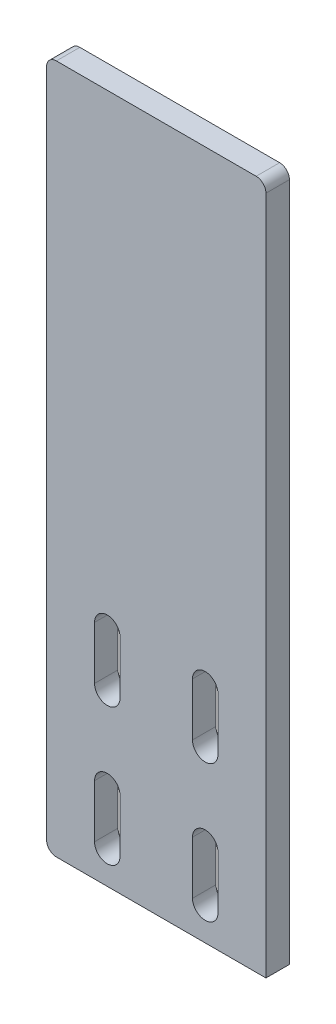
from build123d import *

# Parameters (mm, degrees)
SKETCH1_W           = 112
SKETCH1_H           = 352
BOSS_EXTRUDE1_DEPTH = 12
FILLET1_R           = 5


with BuildPart() as part:
    # Sketch1 → Boss-Extrude1 (new body)
    with BuildSketch(Plane.XY):
        Rectangle(SKETCH1_W, SKETCH1_H)
        with BuildLine():
            Line((-18.5, -62.5), (-18.5, -89.5))
            ThreePointArc((-18.5, -89.5), (-25, -96), (-31.5, -89.5))
            Line((-31.5, -89.5), (-31.5, -62.5))
            ThreePointArc((-31.5, -62.5), (-25, -56), (-18.5, -62.5))
        make_face(mode=Mode.SUBTRACT)
        with BuildLine():
            Line((31.5, -62.5), (31.5, -89.5))
            ThreePointArc((31.5, -89.5), (25, -96), (18.5, -89.5))
            Line((18.5, -89.5), (18.5, -62.5))
            ThreePointArc((18.5, -62.5), (25, -56), (31.5, -62.5))
        make_face(mode=Mode.SUBTRACT)
        with BuildLine():
            Line((-31.5, -132.5), (-31.5, -159.5))
            ThreePointArc((-31.5, -159.5), (-25, -166), (-18.5, -159.5))
            Line((-18.5, -159.5), (-18.5, -132.5))
            ThreePointArc((-18.5, -132.5), (-25, -126), (-31.5, -132.5))
        make_face(mode=Mode.SUBTRACT)
        with BuildLine():
            Line((18.5, -132.5), (18.5, -159.5))
            ThreePointArc((18.5, -159.5), (25, -166), (31.5, -159.5))
            Line((31.5, -159.5), (31.5, -132.5))
            ThreePointArc((31.5, -132.5), (25, -126), (18.5, -132.5))
        make_face(mode=Mode.SUBTRACT)
    extrude(amount=BOSS_EXTRUDE1_DEPTH)

    # Fillet1
    fillet1_edges = [part.edges().sort_by_distance(p)[0] for p in [
        (-56, -176, 6),
        (-56, 176, 6),
        (56, 176, 6),
    ]]
    fillet(fillet1_edges, radius=FILLET1_R)


solid = part.part
